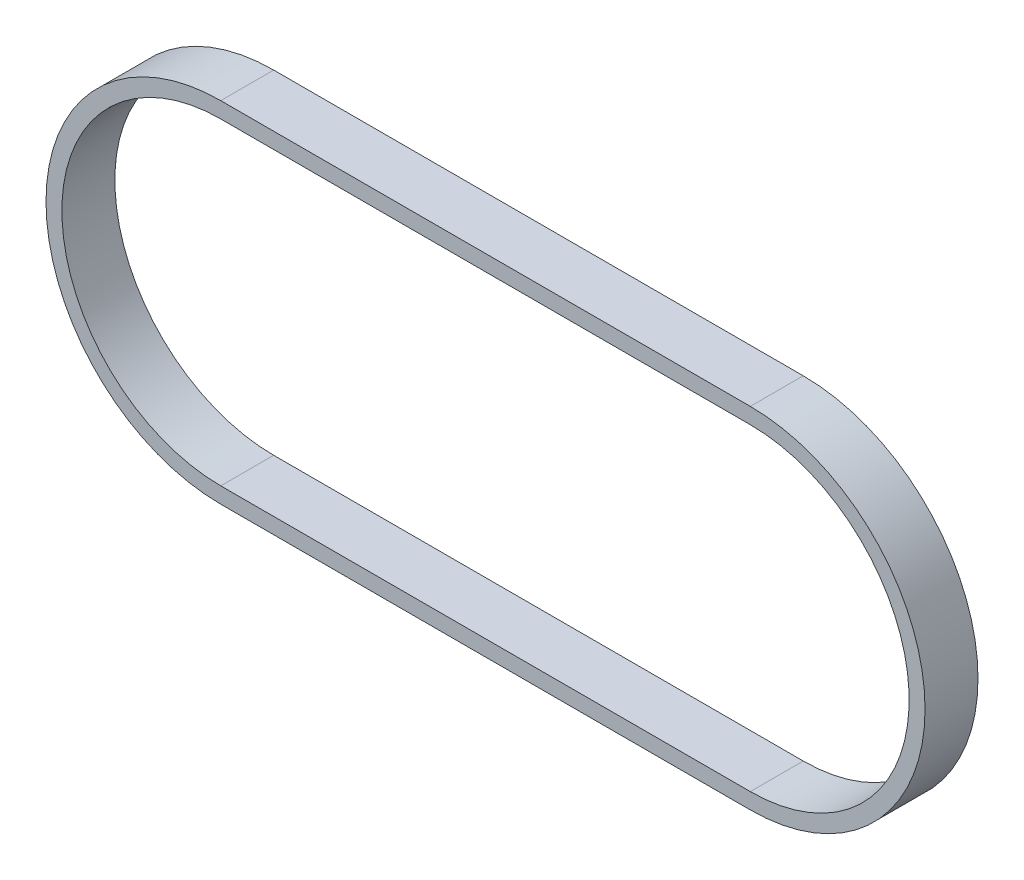
from build123d import *

# Parameters (mm, degrees)
EXTRUDE_1_DEPTH = 5


with BuildPart() as part:
    # 草图1 → 凸台-拉伸1 (new, symmetric)
    with BuildSketch(Plane.XY):
        with BuildLine():
            Line((-50, 33), (50, 33))
            ThreePointArc((50, 33), (83, 0), (50, -33))
            Line((50, -33), (-50, -33))
            ThreePointArc((-50, -33), (-83, 0), (-50, 33))
        make_face()
        with BuildLine():
            Line((-50, 30), (50, 30))
            ThreePointArc((50, 30), (80, 0), (50, -30))
            Line((50, -30), (-50, -30))
            ThreePointArc((-50, -30), (-80, 0), (-50, 30))
        make_face(mode=Mode.SUBTRACT)
    extrude(amount=EXTRUDE_1_DEPTH, both=True)


solid = part.part
